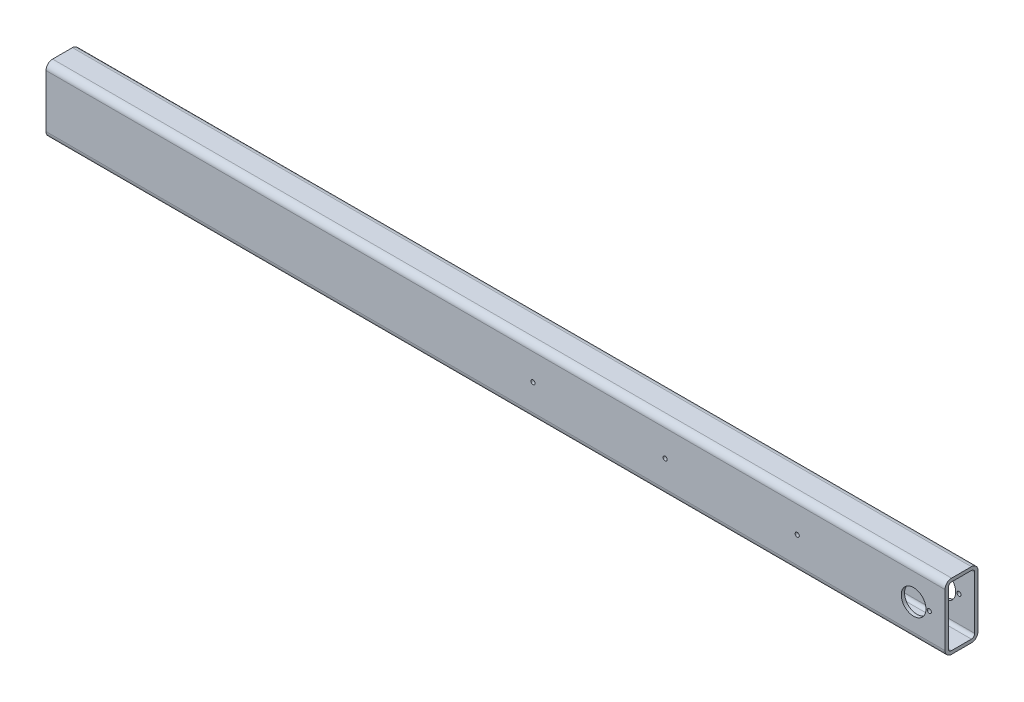
from build123d import *

# Parameters (mm, degrees)
GB_6728_1986_080_X_40_X_4_1_DEPTH = 1089
HOLE_WIZARD_M6_1_D                = 5
SKETCH_4_R                        = 15
CUT_EXTRUDE_1_DEPTH               = 1091.468248048


with BuildPart() as part:
    # Sketch12 → Gb／6728-1986矩形空心型钢 080 X 40 X 4(1) (new body)
    with BuildSketch(Plane(origin=(0, 0, 0), x_dir=(0, 0, -1), z_dir=(1, 0, 0))):
        with BuildLine():
            Line((-12, -40), (12, -40))
            ThreePointArc((12, -40), (17.656854249, -37.656854249), (20, -32))
            Line((20, -32), (20, 32))
            ThreePointArc((20, 32), (17.656854249, 37.656854249), (12, 40))
            Line((12, 40), (-12, 40))
            ThreePointArc((-12, 40), (-17.656854249, 37.656854249), (-20, 32))
            Line((-20, 32), (-20, -32))
            ThreePointArc((-20, -32), (-17.656854249, -37.656854249), (-12, -40))
        make_face()
        with BuildLine():
            Line((-12, -36), (12, -36))
            ThreePointArc((12, -36), (14.828427125, -34.828427125), (16, -32))
            Line((16, -32), (16, 32))
            ThreePointArc((16, 32), (14.828427125, 34.828427125), (12, 36))
            Line((12, 36), (-12, 36))
            ThreePointArc((-12, 36), (-14.828427125, 34.828427125), (-16, 32))
            Line((-16, 32), (-16, -32))
            ThreePointArc((-16, -32), (-14.828427125, -34.828427125), (-12, -36))
        make_face(mode=Mode.SUBTRACT)
    extrude(amount=GB_6728_1986_080_X_40_X_4_1_DEPTH)

    # M6 螺纹孔1 (through all)
    with Locations(Plane(origin=(0, 0, -20), x_dir=(-1, 0, 0), z_dir=(0, 0, -1))):
        with Locations((-590, 0), (-750, 0), (-910, 0), (-1070, 0)):
            Hole(HOLE_WIZARD_M6_1_D / 2)

    # 草图4 → 切除-拉伸1 (cut, through all)
    with BuildSketch(Plane.XY.offset(20)):
        with Locations((1051, 0)):
            Circle(SKETCH_4_R)
    extrude(amount=-CUT_EXTRUDE_1_DEPTH, mode=Mode.SUBTRACT)


solid = part.part
